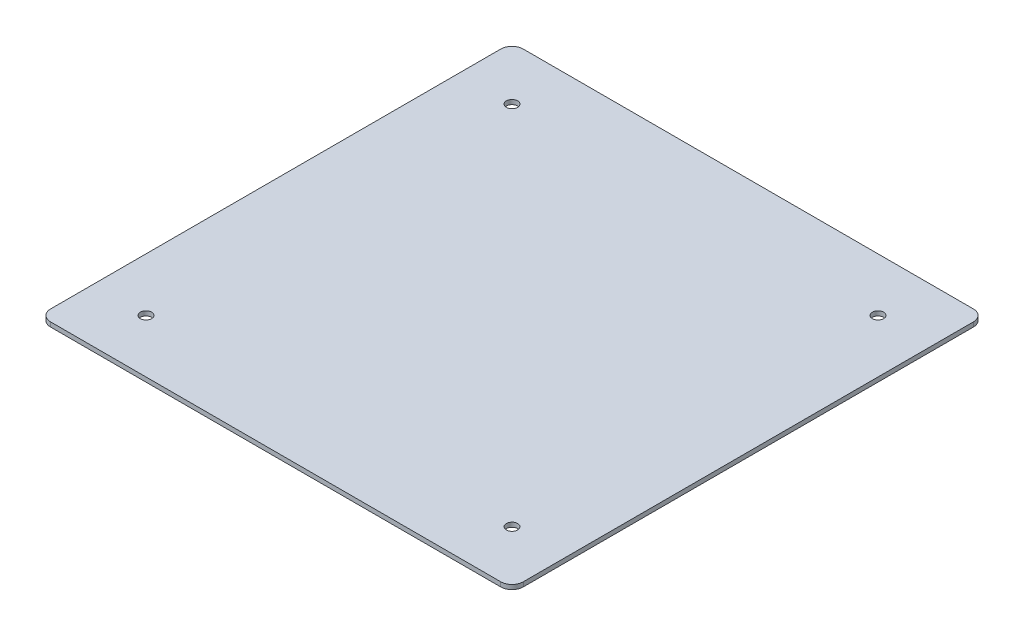
from build123d import *

# Parameters (mm, degrees)
SKETCH_1_W            = 210
SKETCH_1_H            = 210
EXTRUDE_1_DEPTH       = 2
HOLE_WIZARD_5_0_5_1_D = 5
FILLET_1_R            = 5


with BuildPart() as part:
    # 草图1 → 凸台-拉伸1 (new body)
    with BuildSketch(Plane(origin=(0, 0, 0), x_dir=(1, 0, 0), z_dir=(0, 1, 0))):
        Rectangle(SKETCH_1_W, SKETCH_1_H)
    extrude(amount=EXTRUDE_1_DEPTH)

    # Ø5.0 (5) 直径孔1 (through all)
    with Locations(Plane(origin=(0, 2, 0), x_dir=(1, 0, 0), z_dir=(0, 1, 0))):
        with Locations((-81.317279836, -81.317279836), (-81.317279836, 81.317279836), (81.317279836, 81.317279836), (81.317279836, -81.317279836)):
            Hole(HOLE_WIZARD_5_0_5_1_D / 2)

    # 圆角1
    fillet_1_edges = [part.edges().sort_by_distance(p)[0] for p in [
        (105, 1, 105),
        (-105, 1, 105),
        (-105, 1, -105),
        (105, 1, -105),
    ]]
    fillet(fillet_1_edges, radius=FILLET_1_R)


solid = part.part
